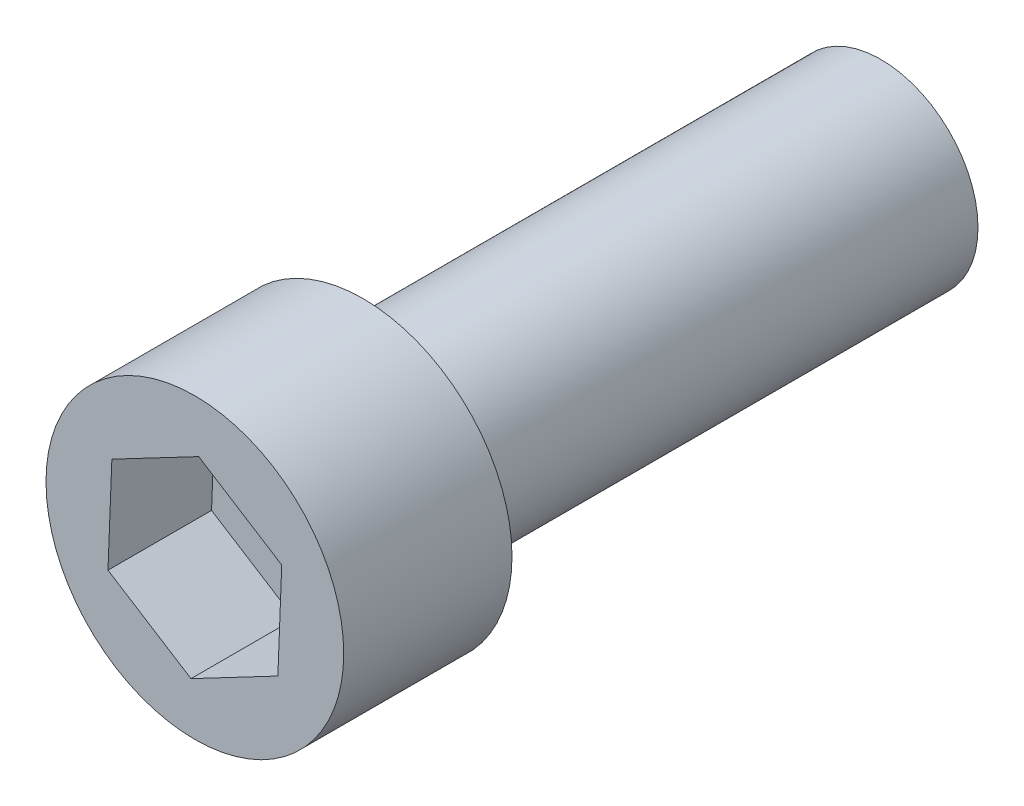
from build123d import *

# Parameters (mm, degrees)
SKETCH1_R           = 7.5
BOSS_EXTRUDE1_DEPTH = 40
SKETCH2_R           = 11.5
BOSS_EXTRUDE2_DEPTH = 13
CUT_EXTRUDE1_DEPTH  = 8


with BuildPart() as part:
    # Sketch1 → Boss-Extrude1 (new body)
    with BuildSketch(Plane.XY):
        Circle(SKETCH1_R)
    extrude(amount=BOSS_EXTRUDE1_DEPTH)

    # Sketch2 → Boss-Extrude2 (add)
    with BuildSketch(Plane.XY.offset(40)):
        with Locations(Location((0, 0, 0), (0, 0, 180))):
            Circle(SKETCH2_R)
    extrude(amount=BOSS_EXTRUDE2_DEPTH)

    # Sketch3 → Cut-Extrude1 (cut)
    with BuildSketch(Plane.XY.offset(53)):
        Polygon((6.412132048, -4.047977261), (6.711717166, 3.529080616), (0.299585118, 7.577057877), (-6.412132048, 4.047977261), (-6.711717166, -3.529080616), (-0.299585118, -7.577057877), align=None)
    extrude(amount=-CUT_EXTRUDE1_DEPTH, mode=Mode.SUBTRACT)


solid = part.part
